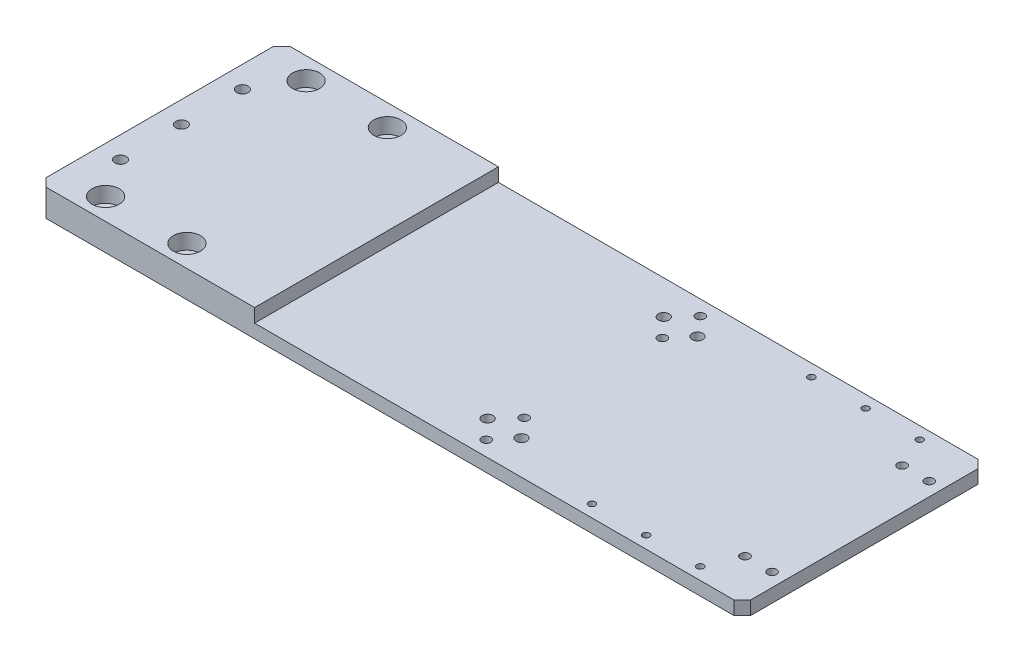
SolidWorks part; units mm, degrees
material "A6061 T6"
ref_plane "前视基准面" through (0, 0, 0) normal (0, 0, 1) x (1, 0, 0)
ref_plane "上视基准面" through (0, 0, 0) normal (0, 1, 0) x (1, 0, 0)
ref_plane "右视基准面" through (0, 0, 0) normal (1, 0, 0) x (0, 0, -1)
sketch "草图1" plane through (0, 0, 0) normal (0, 1, 0) x (1, 0, 0)
  line L1 (-130, 45) -> (130, 45)
  line L2 (-130, 45) -> (-130, -45)
  line L3 (-130, -45) -> (130, -45)
  line L4 (130, 45) -> (130, -45)
  line L5 (-130, 45) -> (130, -45) construction
  line L6 (-130, -45) -> (130, 45) construction
  point P0 (0, 0)
  dimension "D1" = 260
  dimension "D2" = 90
extrude "凸台-拉伸1" add sketch "草图1" along normal blind 10
chamfer "倒角1" distance 3 angle 45 4 edges at (-130, 5, -45) (130, 5, -45) (130, 5, 45) (-130, 5, 45)
hole_wizard "打孔尺寸(%根据)内六角圆柱头螺钉的类型1" positions "草图2" profile "草图3" counterbore size "M5" standard "GB"
sketch "草图2" plane through (0, 10, 0) normal (0, 1, 0) x (1, 0, 0)
  line L0 (-127, -45) -> (127, -45) construction
  line L1 (-130, 42) -> (-130, -42) construction
  point P0 (-83, 37)
  point P3 (-113, 37)
  point P6 (-83, -37)
  point P9 (-113, -37)
  dimension "D1" = 30
  dimension "D2" = 8
  dimension "D3" = 74
  dimension "D4" = 17
sketch "草图3" plane through (-83, 10, -37) normal (1, 0, 0) x (0, 0, 1)
  line L0 (0, 0) -> (0, 11.7524)
  line L1 (0, 11.7524) -> (2.75, 10.1)
  line L2 (2.75, 10.1) -> (2.75, 5.7)
  line L3 (2.75, 5.7) -> (5, 5.7)
  line L4 (5, 5.7) -> (5, 0)
  line L5 (5, 0) -> (0, 0)
  line L10 (0, 11.7524) -> (-2.75, 10.1) construction
  line L11 (0, -6.35) -> (0, 107.95) construction
  dimension "孔直径" = 5.5
  dimension "孔深度" = 10.1
  dimension "柱形沉头孔直径" = 10
  dimension "柱形沉头孔深度" = 5.7
  dimension "导头角度" = 118
hole_wizard "打孔尺寸(%根据)内六角圆柱头螺钉的类型2" positions "草图4" profile "草图5" counterbore size "M4" standard "GB"
sketch "草图4" plane through (0, 0, 0) normal (0, -1, 0) x (-1, 0, 0)
  point P0 (-110, -17.25)
  point P3 (-110, 17.25)
  point P6 (-95, -17.25)
  point P9 (-95, 17.25)
  point P12 (-80, -17.25)
  point P15 (-80, 17.25)
sketch "草图5" plane through (110, 0, 17.25) normal (1, 0, 0) x (0, 0, -1)
  line L0 (0, 0) -> (0, 21.3519)
  line L1 (0, 21.3519) -> (2.25, 20)
  line L2 (2.25, 20) -> (2.25, 4.6)
  line L3 (2.25, 4.6) -> (4, 4.6)
  line L4 (4, 4.6) -> (4, 0)
  line L5 (4, 0) -> (0, 0)
  line L10 (0, 21.3519) -> (-2.25, 20) construction
  line L11 (0, -6.35) -> (0, 107.95) construction
  dimension "孔直径" = 4.5
  dimension "孔深度" = 20
  dimension "柱形沉头孔直径" = 8
  dimension "柱形沉头孔深度" = 4.6
  dimension "导头角度" = 118
hole_wizard "M5 螺纹孔1" positions "草图6" profile "草图7" tap size "M5" standard "GB"
sketch "草图6" plane through (0, 10, 0) normal (0, 1, 0) x (1, 0, 0)
  point P0 (-122, 22.5)
  point P3 (-122, 0)
  point P6 (-122, -22.5)
sketch "草图7" plane through (-122, 10, -22.5) normal (1, 0, 0) x (0, 0, 1)
  line L0 (0, 0) -> (0, 13.6618)
  line L1 (0, 13.6618) -> (2.1, 12.4)
  line L2 (2.1, 12.4) -> (2.1, 0)
  line L5 (2.1, 0) -> (0, 0)
  line L10 (0, 13.6618) -> (-2.1, 12.4) construction
  line L11 (0, -6.35) -> (0, 107.95) construction
  dimension "螺纹孔钻头直径" = 4.2
  dimension "螺纹孔钻头深度" = 12.4
  dimension "导头角度" = 118
cosmetic thread "孔螺蚊线1"
cosmetic thread "孔螺蚊线2"
cosmetic thread "孔螺蚊线3"
sketch "草图8" plane through (0, 10, 0) normal (0, 1, 0) x (1, 0, 0)
  line L0 (127, 45) -> (-127, 45) construction
  line L1 (-50, 45) -> (130, 45)
  line L2 (-50, 45) -> (-50, -45)
  line L3 (-50, -45) -> (130, -45)
  line L4 (130, 45) -> (130, -45)
  line L5 (-127, -45) -> (127, -45) construction
  line L6 (130, -42) -> (130, 42) construction
  dimension "D1" = 180
extrude "切除-拉伸1" cut sketch "草图8" against normal blind 5
hole_wizard "M3 螺纹孔1" positions "草图9" profile "草图10" tap size "M3" standard "GB"
sketch "草图9" plane through (0, 5, 0) normal (0, 1, 0) x (1, 0, 0)
  point P0 (110, -40.5)
  point P3 (90, -40.5)
  point P6 (70, -40.5)
  point P9 (110, 40.5)
  point P12 (90, 40.5)
  point P15 (70, 40.5)
sketch "草图10" plane through (110, 5, 40.5) normal (1, 0, 0) x (0, 0, 1)
  line L0 (0, 0) -> (0, 8.2511)
  line L1 (0, 8.2511) -> (1.25, 7.5)
  line L2 (1.25, 7.5) -> (1.25, 0)
  line L5 (1.25, 0) -> (0, 0)
  line L10 (0, 8.2511) -> (-1.25, 7.5) construction
  line L11 (0, -6.35) -> (0, 107.95) construction
  dimension "螺纹孔钻头直径" = 2.5
  dimension "螺纹孔钻头深度" = 7.5
  dimension "导头角度" = 118
cosmetic thread "孔螺蚊线4"
cosmetic thread "孔螺蚊线5"
cosmetic thread "孔螺蚊线6"
cosmetic thread "孔螺蚊线7"
cosmetic thread "孔螺蚊线8"
cosmetic thread "孔螺蚊线9"
hole_wizard "M4 螺纹孔1" positions "草图11" profile "草图12" tap size "M4" standard "GB"
sketch "草图11" plane through (0, 5, 0) normal (0, 1, 0) x (1, 0, 0)
  point P0 (115, -29)
  point P3 (125, -29)
  point P6 (115, 29)
  point P9 (125, 29)
sketch "草图12" plane through (115, 5, 29) normal (1, 0, 0) x (0, 0, 1)
  line L0 (0, 0) -> (0, 20.9914)
  line L1 (0, 20.9914) -> (1.65, 20)
  line L2 (1.65, 20) -> (1.65, 0)
  line L5 (1.65, 0) -> (0, 0)
  line L10 (0, 20.9914) -> (-1.65, 20) construction
  line L11 (0, -6.35) -> (0, 107.95) construction
  dimension "螺纹孔钻头直径" = 3.3
  dimension "螺纹孔钻头深度" = 20
  dimension "导头角度" = 118
cosmetic thread "孔螺蚊线10"
cosmetic thread "孔螺蚊线11"
cosmetic thread "孔螺蚊线12"
cosmetic thread "孔螺蚊线13"
hole_wizard "M4 螺纹孔2" positions "草图13" profile "草图14" tap size "M4" standard "GB"
sketch "草图13" plane through (0, 10, 0) normal (0, 1, 0) x (1, 0, 0)
  point P0 (30, -25.5)
  point P3 (30, -39.5)
  point P5 (30, 25.5)
  point P8 (30, 39.5)
sketch "草图14" plane through (30, 10, 25.5) normal (1, 0, 0) x (0, 0, 1)
  line L0 (0, 0) -> (0, 20.9914)
  line L1 (0, 20.9914) -> (1.65, 20)
  line L2 (1.65, 20) -> (1.65, 0)
  line L5 (1.65, 0) -> (0, 0)
  line L10 (0, 20.9914) -> (-1.65, 20) construction
  line L11 (0, -6.35) -> (0, 107.95) construction
  dimension "螺纹孔钻头直径" = 3.3
  dimension "螺纹孔钻头深度" = 20
  dimension "导头角度" = 118
cosmetic thread "孔螺蚊线14"
cosmetic thread "孔螺蚊线15"
cosmetic thread "孔螺蚊线16"
cosmetic thread "孔螺蚊线17"
hole_wizard "大小mm 暗销孔1" positions "草图15" profile "草图16" hole size "Ø4.0" standard "GB"
sketch "草图15" plane through (0, 5, 0) normal (0, 1, 0) x (1, 0, 0)
  point P0 (23.5, -32.5)
  point P3 (36, -32.5)
  point P6 (23.5, 32.5)
  point P9 (36, 32.5)
sketch "草图16" plane through (23.5, 5, 32.5) normal (1, 0, 0) x (0, 0, 1)
  line L0 (0, 0) -> (0, 21.2017)
  line L1 (0, 21.2017) -> (2, 20)
  line L2 (2, 20) -> (2, 0)
  line L5 (2, 0) -> (0, 0)
  line L10 (0, 21.2017) -> (-2, 20) construction
  line L11 (0, -6.35) -> (0, 107.95) construction
  dimension "孔直径" = 4
  dimension "孔深度" = 20
  dimension "导头角度" = 118
